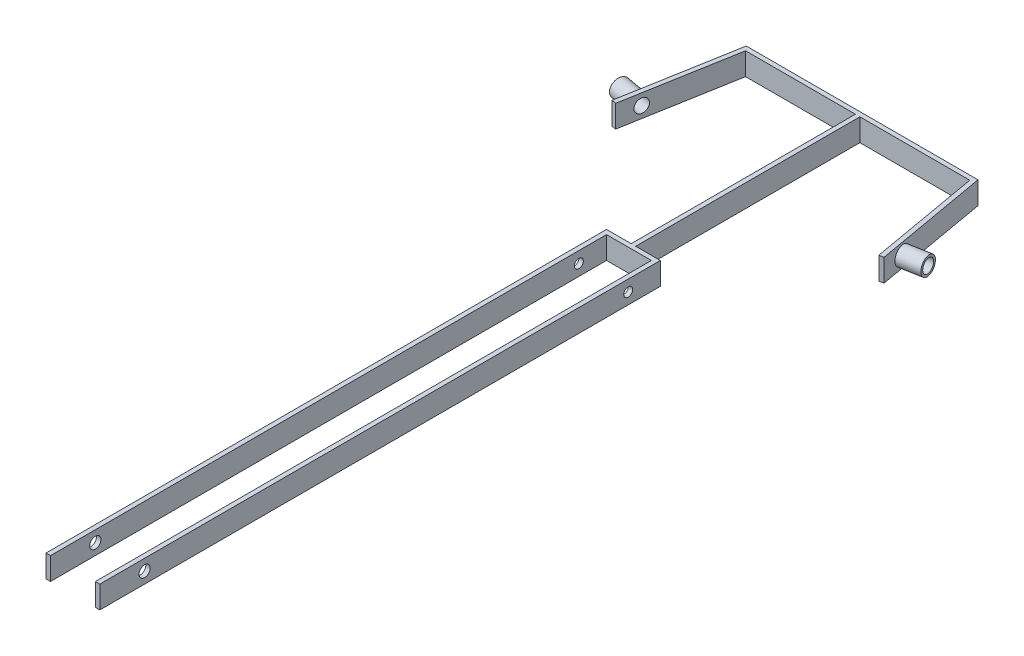
from build123d import *

# Parameters (mm, degrees)
EXTRUDE_1_DEPTH     = 10
SKETCH_3_W          = 100
SKETCH_3_H          = 10
EXTRUDE_2_DEPTH     = 1
EXTRUDE_3_DEPTH     = 10
SKETCH_6_R          = 4
SKETCH_6_R_2        = 3
EXTRUDE_4_DEPTH     = 10
CUT_EXTRUDE_START   = -20
SKETCH_7_R          = 3
CUT_EXTRUDE_1_DEPTH = 20
SKETCH_9_R          = 2.5
CUT_EXTRUDE_2_DEPTH = 274
SKETCH_10_R         = 2
CUT_EXTRUDE_3_DEPTH = 45


with BuildPart() as part:
    # 草图1 → 凸台-拉伸1 (new body)
    with BuildSketch(Plane(origin=(0, 0, 0), x_dir=(1, 0, 0), z_dir=(0, 1, 0))):
        Polygon((-10, -248), (-10, 0), (10, 0), (10, -248), (12, -248), (12, 2), (-12, 2), (-12, -248), align=None)
    extrude(amount=EXTRUDE_1_DEPTH)

    # 草图3 → 凸台-拉伸2 (add, symmetric)
    with BuildSketch(Plane(origin=(0, 0, 0), x_dir=(0, 0, -1), z_dir=(1, 0, 0))):
        with Locations((52, 5)):
            Rectangle(SKETCH_3_W, SKETCH_3_H)
    extrude(amount=EXTRUDE_2_DEPTH, both=True)

    # 草图4 → 凸台-拉伸3 (add)
    with BuildSketch(Plane(origin=(0, 0, 0), x_dir=(1, 0, 0), z_dir=(0, 1, 0))):
        Polygon((-50, 102), (50, 102), (58.682408883, 52.759612349), (60.652024389, 53.106908705), (51.678199262, 104), (-51.678199262, 104), (-60.652024389, 53.106908705), (-58.682408883, 52.759612349), align=None)
    extrude(amount=EXTRUDE_3_DEPTH)

    # 草图6 → 凸台-拉伸4 (add)
    with BuildSketch(Plane(origin=(-67.904958335, 0, -11.973476278), x_dir=(-0.17364817766693408, 0, 0.9848077530122076), z_dir=(-0.9848077530122076, 0, -0.17364817766693408))):
        with Locations(Location((-51.767981924, 5, 0), (0, 0, 180))):
            Circle(SKETCH_6_R)
        with Locations((-51.767981924, 5)):
            Circle(SKETCH_6_R_2, mode=Mode.SUBTRACT)
    extrude_4 = extrude(amount=EXTRUDE_4_DEPTH)

    # 草图7 → 切除-拉伸1 (cut)
    with BuildSketch(Plane(origin=(-67.904958335, 0, -11.973476278), x_dir=(-0.17364817766693408, 0, 0.9848077530122076), z_dir=(-0.9848077530122076, 0, -0.17364817766693408)).offset(CUT_EXTRUDE_START)):
        with Locations((-51.767981924, 5)):
            Circle(SKETCH_7_R)
    cut_extrude_1 = extrude(amount=CUT_EXTRUDE_1_DEPTH, mode=Mode.SUBTRACT)

    # 镜向1: 凸台-拉伸4, 切除-拉伸1 across plane
    add(extrude_4.mirror(Plane(origin=(0, 0, 0), x_dir=(0, 0, 1), z_dir=(1, 0, 0))))
    add(cut_extrude_1.mirror(Plane(origin=(0, 0, 0), x_dir=(0, 0, 1), z_dir=(1, 0, 0))), mode=Mode.SUBTRACT)

    # 草图9 → 切除-拉伸2 (cut)
    with BuildSketch(Plane.ZY.offset(12)):
        with Locations((228, 5)):
            Circle(SKETCH_9_R)
    extrude(amount=-CUT_EXTRUDE_2_DEPTH, mode=Mode.SUBTRACT)

    # 草图10 → 切除-拉伸3 (cut)
    with BuildSketch(Plane.ZY.offset(12)):
        with Locations((12.339097651, 5)):
            Circle(SKETCH_10_R)
    extrude(amount=-CUT_EXTRUDE_3_DEPTH, mode=Mode.SUBTRACT)


solid = part.part
